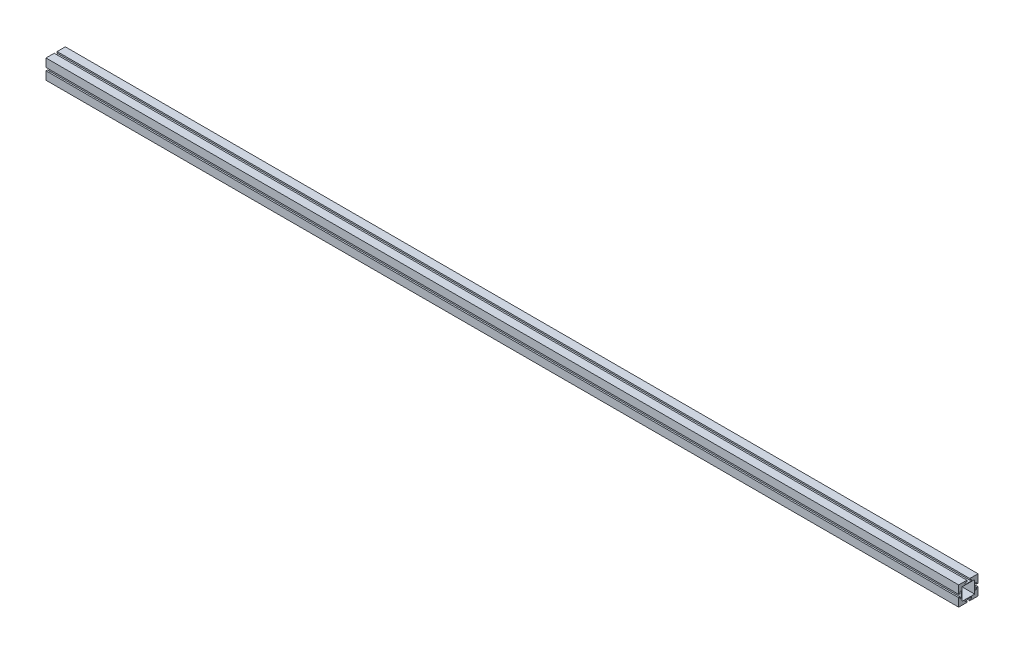
from build123d import *

# Parameters (mm, degrees)
SKETCH1_W           = 26
SKETCH1_H           = 26
BOSS_EXTRUDE1_DEPTH = 1890


with BuildPart() as part:
    # Sketch1 → Boss-Extrude1 (new body)
    with BuildSketch(Plane(origin=(0, 0, 0), x_dir=(0, 0, -1), z_dir=(1, 0, 0))):
        Polygon((-20, -20), (-3, -20), (-3, -17), (-6.5, -17), (-6.5, -14), (6.5, -14), (6.5, -17), (3, -17), (3, -20), (20, -20), (20, -3), (17, -3), (17, -6.5), (14, -6.5), (14, 6.5), (17, 6.5), (17, 3), (20, 3), (20, 20), (3, 20), (3, 17), (6.5, 17), (6.5, 14), (-6.5, 14), (-6.5, 17), (-3, 17), (-3, 20), (-20, 20), (-20, 3), (-17, 3), (-17, 6.5), (-14, 6.5), (-14, -6.5), (-17, -6.5), (-17, -3), (-20, -3), align=None)
        Rectangle(SKETCH1_W, SKETCH1_H, mode=Mode.SUBTRACT)
    extrude(amount=BOSS_EXTRUDE1_DEPTH)


solid = part.part
